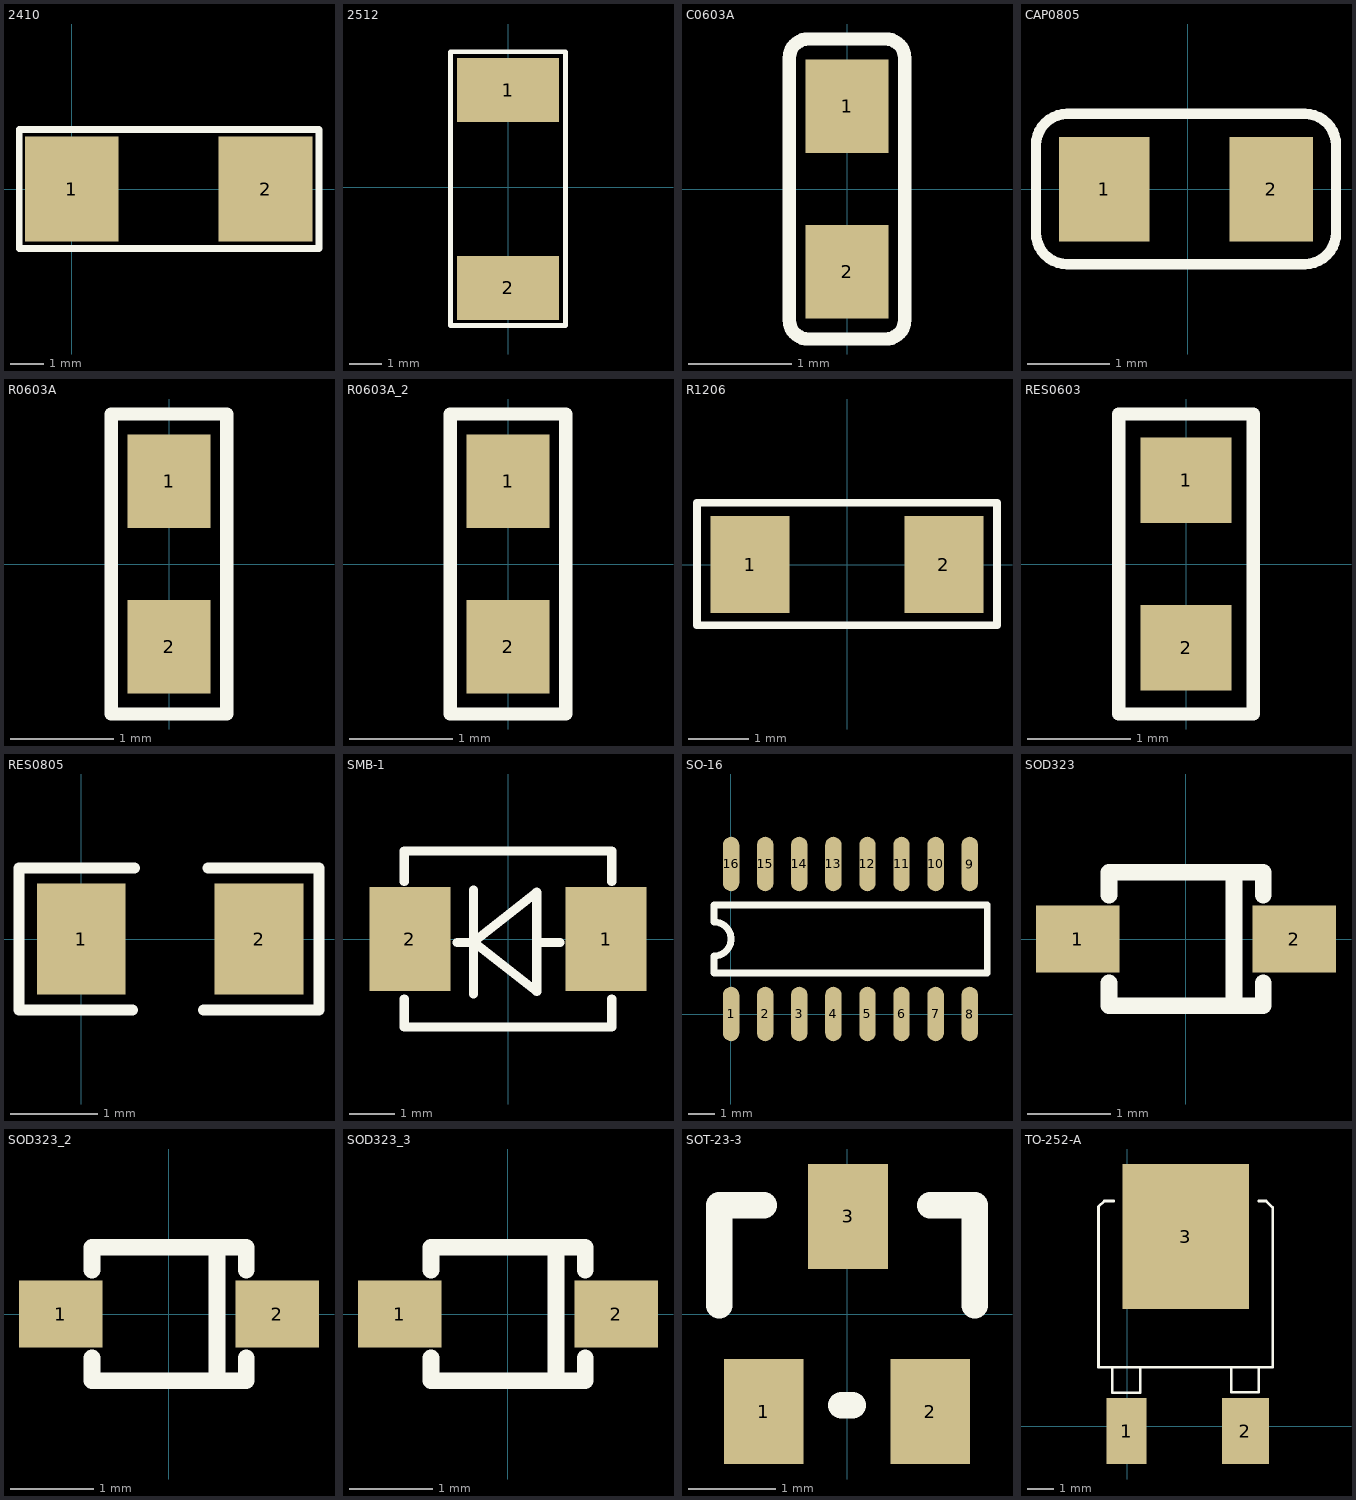
[diagram p0: the footprints below, top view; thin cyan lines are the x and y axes]
# Altium footprint library MISC86331.PcbLib: 18 footprints (part 1 of 2)
Each footprint in its own frame and in the unit in brackets; x right, y up, seen from the top. Pads: shape width x height; smd on the part's side, far side on the other; paste and mask are expansions set on the pad; w line width, h text height; cw(c..) or ccw(c..) is an arc to the next point about the centre after c.

## 2410 [mm]
pads (2):
  rect 2.8x3.15 smd: 1(0.001,0.001) 2(5.8,0)
Top Overlay:
  lines w0.2: 1.2,-1.777 7.4,-1.777 7.4,1.779 4.5,1.779 ; 1.3,-1.777 -1.569,-1.777 -1.569,1.779 4.8,1.779

## 2512 [mm]
height 2.5
pads (2):
  rect 3.2x2 smd: 1(0,3.05) 2(0,-3.15)
Top Overlay:
  lines w0.15: -1.802,-4.325 1.801,-4.325 1.801,4.25 -1.802,4.25 -1.802,-4.325

## C0603A [mm]
pads (2):
  rect 0.8x0.9 smd: 1(0,0.8) 2(0,-0.8)
Top Overlay:
  lines w0.13: -0.56,-1.25 -0.56,0.544 ; -0.56,0.485 -0.56,1.25 ; -0.557,-1.268 ccw(c-0.375,-1.268) -0.375,-1.45 0.375,-1.45 ccw(c0.375,-1.268) 0.557,-1.268 ; -0.557,1.268 cw(c-0.375,1.268) -0.375,1.45 ; -0.4,1.45 0.378,1.45 ; 0.375,1.45 cw(c0.375,1.268) 0.557,1.268 ; 0.56,-1.25 0.56,0.534 ; 0.56,0.485 0.56,1.25

## CAP0805 [mil]
height 100
pads (2):
  rect 43.31x50 smd: 1(-40,0)
  rect 40x50 smd: 2(40,0)
Top Overlay:
  lines w5: 56,-35.96 -57.66,-35.96 cw(c-57.66,-21) -72.62,-21 -72.62,21 cw(c-57.66,21) -57.66,35.96 56,35.96 ; 56,-35.92 ccw(c56,-20.96) 70.96,-20.96 70.96,21.04 ccw(c56,21.04) 56,36
3D body "0805 SMD Capacitor.STEP": height 34.72, standoff 3.94, extent -39.36,-24.6 39.38,24.61

## R0603A [mm]
pads (2):
  rect 0.8x0.9 smd: 1(0,0.8) 2(0,-0.8)
Top Overlay:
  lines w0.13: -0.56,-1.352 -0.56,-1.35 ; -0.56,0.471 -0.56,1.45 0.56,1.45 0.56,0.471 ; -0.56,0.53 -0.56,-1.45 0.56,-1.45 0.56,0.505

## R0603A_2 [mm]
pads (2):
  rect 0.8x0.9 smd: 1(0,0.8) 2(0,-0.8)
Top Overlay:
  lines w0.13: -0.56,-1.352 -0.56,-1.35 ; -0.56,0.471 -0.56,1.45 0.56,1.45 0.56,0.471 ; -0.56,0.53 -0.56,-1.45 0.56,-1.45 0.56,0.505

## R1206 [mm]
pads (2):
  rect 1.3x1.6 smd: 1(-1.6,0) 2(1.6,0)
Top Overlay:
  lines w0.127: -2.475,-1 -2.475,1.019 2.475,1.019 2.475,-1 -2.475,-1

## RES0603 [mm] "CAP0402"
height 3.35
pads (2):
  rect 0.88x0.83 smd mask+0: 1(0,0.81) 2(0,-0.81)
Top Overlay:
  lines w0.127: 0.64,-1.45 -0.65,-1.45 -0.65,-0.4 -0.65,1.45 0.65,1.45 0.65,-0.44 ; 0.65,-1.45 0.65,-0.4
3D body "0603res.stp": height 0.3, standoff 0, extent -0.4,-0.83 0.4,0.77

## RES0805 [mil]
height 100
pads (2):
  rect 40x50 smd: 1(0,0) 2(80,0)
Top Overlay:
  lines w5: 23,-32 -28,-32 -28,32 24,32 ; 55,-32 107,-32 107,32 57,32
3D body "RES0805.STEP": height 3.94, standoff -12.2, extent 0.63,-25 79.37,24.21

## SMB-1 [mm]
pads (2):
  rect 1.8x2.3 smd: 1(2.175,0) 2(-2.175,0)
Top Overlay:
  lines w0.2: -2.3,-1.325 -2.3,-1.95 2.3,-1.95 2.3,-1.325 ; -2.3,1.275 -2.3,1.95 2.3,1.95 2.3,1.275 ; -1.125,-0.075 -0.762,-0.075 -0.762,1.086 ; -0.762,-1.214 -0.762,-0.064 ; 0.65,-0.075 1.15,-0.075 ; -0.762,-0.064 0.638,1.036 0.638,-1.164 -0.762,-0.064

## SO-16 [mil]
height 98.43
pads (16):
  oval 24x80 smd: 1(0.36,0.36) 2(50.36,0.36) 3(100.36,0.36) 4(150.36,0.36) 5(200.36,0.36) 6(250.36,0.36) 7(300.36,0.36) 8(350.35,0.35) 9(350.35,220.35) 10(300.36,220.36) 11(250.36,220.36) 12(200.36,220.36) 13(150.36,220.36) 14(100.36,220.36) 15(50.36,220.36) 16(0.36,220.36)
Top Overlay:
  lines w9.84: -24.64,85.36 -24.64,60.36 375.98,60.36 375.98,160.36 -24.64,160.36 -24.64,135.36
  lines w10: -24.64,85.36 ccw(c-24.64,110.36) -24.64,135.36

## SOD323 [mm]
height 2.45
pads (2):
  rect 1x0.8 smd: 1(-1.3,0) 2(1.3,0)
Top Overlay:
  lines w0.2: -0.924,-0.525 -0.924,-0.8 0.926,-0.8 0.926,-0.525 ; -0.924,0.525 -0.924,0.8 0.926,0.8 0.926,0.525 ; 0.576,-0.8 0.576,-0.5 0.576,0.8

## SOD323_2 [mm]
pads (2):
  rect 1x0.8 smd: 1(-1.3,0) 2(1.3,0)
Top Overlay:
  lines w0.2: -0.924,-0.525 -0.924,-0.8 0.926,-0.8 0.926,-0.525 ; -0.924,0.525 -0.924,0.8 0.926,0.8 0.926,0.525 ; 0.576,-0.8 0.576,-0.5 0.576,0.8

## SOD323_3 [mm]
pads (2):
  rect 1x0.8 smd: 1(-1.3,0) 2(1.3,0)
Top Overlay:
  lines w0.2: -0.924,-0.525 -0.924,-0.8 0.926,-0.8 0.926,-0.525 ; -0.924,0.525 -0.924,0.8 0.926,0.8 0.926,0.525 ; 0.576,-0.8 0.576,-0.5 0.576,0.8

## SOT-23-3 [mil]
height 98.43
pads (3):
  rect 36x47.24 smd: 1(-37.5,-43.94) 2(37.5,-43.94) 3(0.5,43.94)
Top Overlay:
  lines w12: -57.5,3.94 -57.5,48.94 -37.5,48.94 ; -2.5,-41.06 2.5,-41.06 ; 37.5,48.94 57.5,48.94 57.5,3.94

## TO-252-A [mm]
height 2.5
pads (3):
  rect 1.5x2.5 smd: 1(-0.026,-0.189)
  rect 1.8x2.5 smd: 2(4.484,-0.189)
  rect 4.8x5.5 smd: 3(2.214,7.181)
Top Overlay:
  lines w0.1: -0.561,2.231 -0.561,1.256 0.489,1.256 0.489,2.181 ; -0.511,8.531 -0.869,8.531 -1.086,8.314 -1.086,2.231 5.514,2.231 5.514,8.286 5.269,8.531 4.989,8.531 ; 3.939,2.231 3.939,1.281 4.989,1.281 4.989,2.231
3D body: height 0.5, standoff 0, extent -0.95,8.1 5.25,9.65
3D body: height 0.5, standoff 0, extent -0.6,-0.25 0.45,2.25
3D body: height 0.5, standoff 0, extent 3.9,-0.35 4.95,2.15
3D body: height 0.5, standoff 0, extent 1.6,1.3 2.65,2.55
3D body: height 0.5, standoff 0, extent -0.95,2.3 5.35,8.25
3D body: height 2.5, standoff 0, extent -0.95,8.05 -0.95,8.15